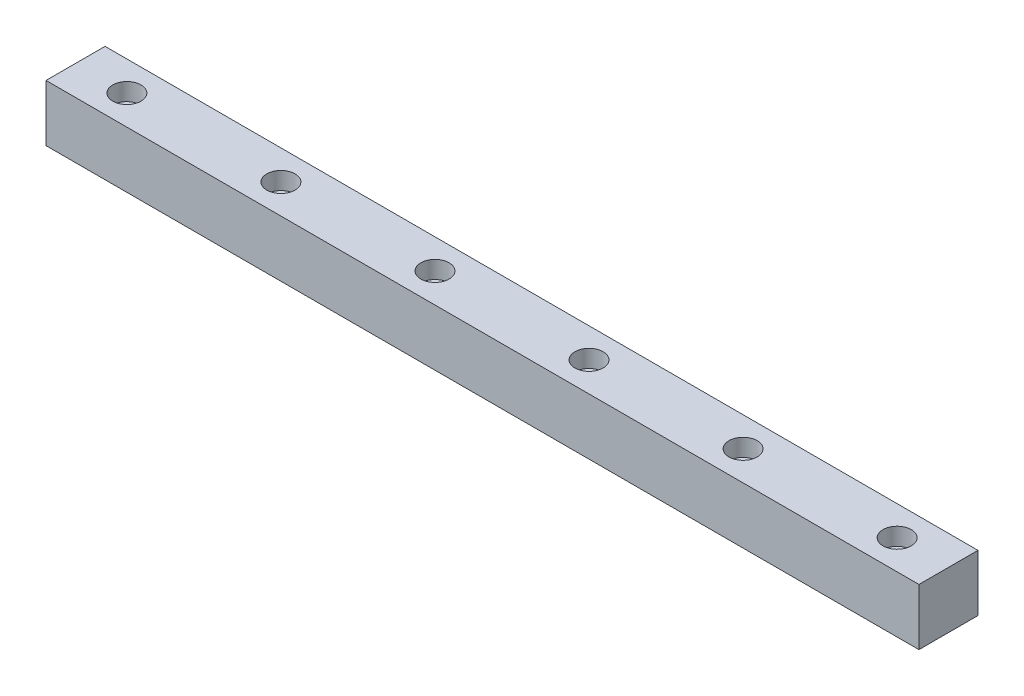
SolidWorks part; units mm, degrees
ref_plane "前视基准面" through (0, 0, 0) normal (0, 0, 1) x (1, 0, 0)
ref_plane "上视基准面" through (0, 0, 0) normal (0, 1, 0) x (1, 0, 0)
ref_plane "右视基准面" through (0, 0, 0) normal (1, 0, 0) x (0, 0, -1)
sketch "草图1" plane through (0, 0, 0) normal (1, 0, 0) x (0, 0, -1)
  line L1 (-11.5, 11) -> (11.5, 11)
  line L2 (-11.5, 11) -> (-11.5, -11)
  line L3 (-11.5, -11) -> (11.5, -11)
  line L4 (11.5, 11) -> (11.5, -11)
  line L5 (-11.5, 11) -> (11.5, -11) construction
  line L6 (-11.5, -11) -> (11.5, 11) construction
  point P0 (0, 0)
  dimension "D1" = 23
  dimension "D2" = 22
extrude "凸台-拉伸1" add sketch "草图1" along normal blind 340
hole_wizard "打孔尺寸(%根据)内六角圆柱头螺钉的类型1" positions "草图2" profile "草图3" counterbore size "M6" standard "GB" end condition through all
sketch "草图2" plane through (0, 11, 0) normal (0, 1, 0) x (1, 0, 0)
  line L0 (0, 11.5) -> (0, -11.5) construction
  point P0 (20, 0)
  dimension "D1" = 20
sketch "草图3" plane through (20, 11, 0) normal (1, 0, 0) x (0, 0, 1)
  line L0 (0, 0) -> (0, 22)
  line L1 (0, 22) -> (3.3, 22)
  line L3 (3.3, 22) -> (3.3, 6.8)
  line L4 (3.3, 6.8) -> (5.5, 6.8)
  line L5 (5.5, 6.8) -> (5.5, 0)
  line L7 (5.5, 0) -> (0, 0)
  line L11 (0, -6.35) -> (0, 107.95) construction
  dimension "通孔孔直径" = 6.6
  dimension "通孔孔深度" = 22
  dimension "柱形沉头孔直径" = 11
  dimension "柱形沉头孔深度" = 6.8
pattern_linear "阵列(线性)2" count 6 spacing 60 along (1, 0, 0) of "打孔尺寸(%根据)内六角圆柱头螺钉的类型1"
